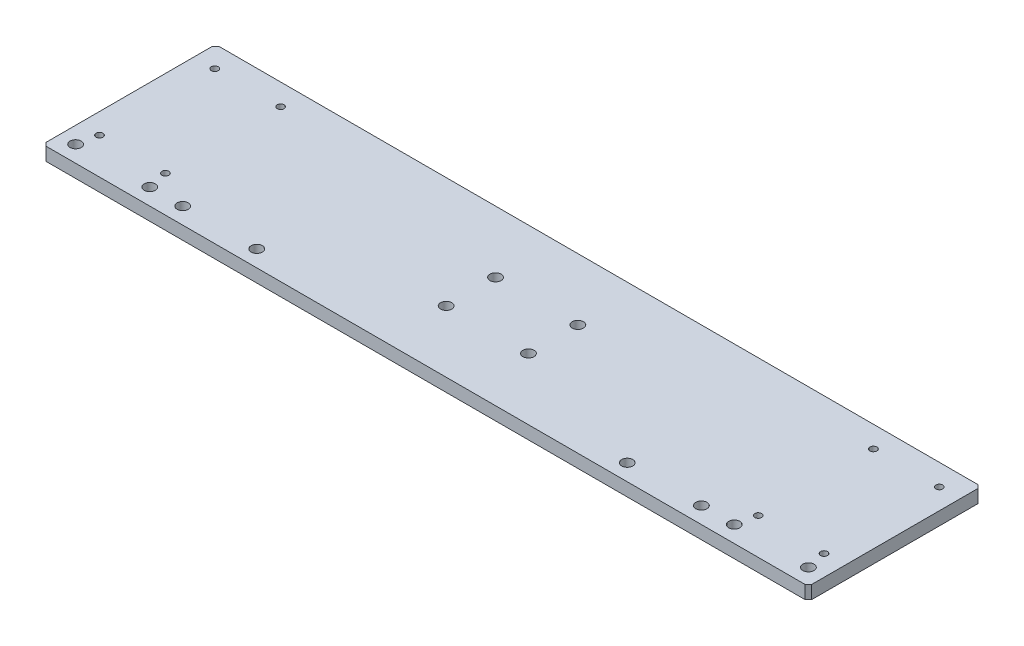
from build123d import *

# Parameters (mm, degrees)
SKETCH_1_W              = 465
SKETCH_1_H              = 105
EXTRUDE_1_DEPTH         = 4
CHAMFER_1_SIZE          = 2
HOLE_WIZARD_M5_1_D      = 4.2
HOLE_WIZARD_6_8_6_8_1_D = 6.8
HOLE_WIZARD_M8_1_D      = 6.8


with BuildPart() as part:
    # 草图1 → 凸台-拉伸1 (new, symmetric)
    with BuildSketch(Plane(origin=(0, 0, 0), x_dir=(1, 0, 0), z_dir=(0, 1, 0))):
        Rectangle(SKETCH_1_W, SKETCH_1_H)
    extrude(amount=EXTRUDE_1_DEPTH, both=True)

    # 倒角1
    chamfer_1_edges = [part.edges().sort_by_distance(p)[0] for p in [
        (232.5, 0, 52.5),
        (-232.5, 0, 52.5),
        (-232.5, 0, -52.5),
        (232.5, 0, -52.5),
    ]]
    chamfer(chamfer_1_edges, length=CHAMFER_1_SIZE)

    # M5 螺纹孔1 (through all)
    with Locations(Plane(origin=(0, 4, 0), x_dir=(1, 0, 0), z_dir=(0, 1, 0))):
        with Locations((-220, 39.5), (-180, 39.5), (-180, -30.5), (-220, -30.5), (220, -30.5), (180, -30.5), (180, 39.5), (220, 39.5)):
            Hole(HOLE_WIZARD_M5_1_D / 2)

    # Ø6.8 (6.8) 直径孔1 (through all)
    with Locations(Plane(origin=(0, 4, 0), x_dir=(1, 0, 0), z_dir=(0, 1, 0))):
        with Locations((25, -15), (25, 15), (-25, 15), (-25, -15)):
            Hole(HOLE_WIZARD_6_8_6_8_1_D / 2)

    # M8 螺纹孔1 (through all)
    with Locations(Plane(origin=(0, 4, 0), x_dir=(1, 0, 0), z_dir=(0, 1, 0))):
        with Locations((222.5, -42.5), (177.5, -42.5), (-177.5, -42.5), (-222.5, -42.5), (157.5, -42.5), (112.5, -42.5), (-112.5, -42.5), (-157.5, -42.5)):
            Hole(HOLE_WIZARD_M8_1_D / 2)


solid = part.part
